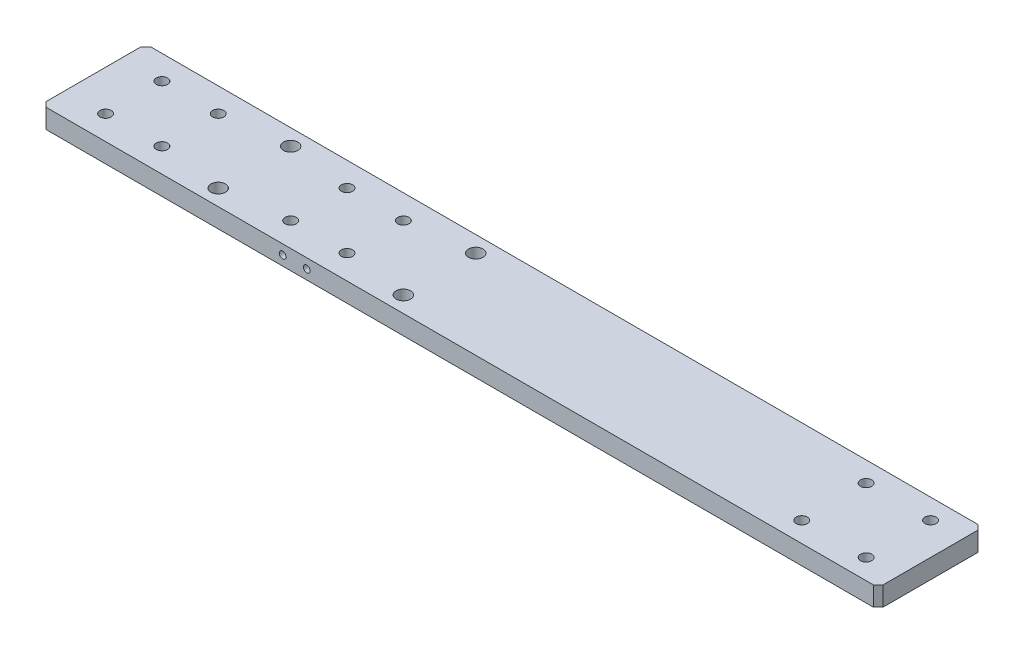
from build123d import *

# Parameters (mm, degrees)
SKETCH_2_W             = 520
SKETCH_2_H             = 65
EXTRUDE_1_DEPTH        = 12
HOLE_WIZARD_7_0_7_1_D  = 7
CHAMFER_1_SIZE         = 3
HOLE_WIZARD_9_0_9_2_D  = 9
HOLE_WIZARD_9_0_9_1_D  = 7
PATTERN_LINEAR_1_COUNT = 2
PATTERN_LINEAR_1_PITCH = 115
HOLE_WIZARD_9_0_9_3_D  = 9
HOLE_WIZARD_M5_1_D     = 4.2
HOLE_WIZARD_M5_1_DEPTH = 12.4
HOLE_WIZARD_M5_1_TIP   = 1.2618073
HOLE_WIZARD_M5_2_D     = 4.2
HOLE_WIZARD_M5_2_DEPTH = 12.4
HOLE_WIZARD_M5_2_TIP   = 1.2618073


with BuildPart() as part:
    # 草图2 → 凸台-拉伸1 (new body)
    with BuildSketch(Plane(origin=(0, 0, 0), x_dir=(1, 0, 0), z_dir=(0, 1, 0))):
        Rectangle(SKETCH_2_W, SKETCH_2_H)
    extrude(amount=EXTRUDE_1_DEPTH)

    # Ø7.0 (7) 直径孔1 (through all)
    with Locations(Plane.XZ):
        with Locations((240, -20), (200, -20), (200, 20), (240, 20)):
            Hole(HOLE_WIZARD_7_0_7_1_D / 2)

    # 倒角1
    chamfer_1_edges = [part.edges().sort_by_distance(p)[0] for p in [
        (260, 6, 32.5),
        (-260, 6, 32.5),
        (-260, 6, -32.5),
        (260, 6, -32.5),
    ]]
    chamfer(chamfer_1_edges, length=CHAMFER_1_SIZE)

    # Ø9.0 (9) 直径孔2 (through all)
    with Locations(Plane(origin=(0, 12, 0), x_dir=(1, 0, 0), z_dir=(0, 1, 0))):
        with Locations((-160, -22.5), (-160, 22.5)):
            Hole(HOLE_WIZARD_9_0_9_2_D / 2)

    # Ø9.0 (9) 直径孔1 (through all)
    with Locations(Plane(origin=(0, 12, 0), x_dir=(1, 0, 0), z_dir=(0, 1, 0))):
        with Locations((-235, -17.5), (-235, 17.5), (-200, -17.5), (-200, 17.5)):
            hole_wizard_9_0_9_1 = Hole(HOLE_WIZARD_9_0_9_1_D / 2)

    # 阵列(线性)1: Ø9.0 (9) 直径孔1 ×2
    with Locations(*[(i * PATTERN_LINEAR_1_PITCH, 0, 0) for i in range(1, PATTERN_LINEAR_1_COUNT)]):
        add(hole_wizard_9_0_9_1, mode=Mode.SUBTRACT)

    # Ø9.0 (9) 直径孔3 (through all)
    with Locations(Plane(origin=(0, 12, 0), x_dir=(1, 0, 0), z_dir=(0, 1, 0))):
        with Locations((-45, -22.5), (-45, 22.5)):
            Hole(HOLE_WIZARD_9_0_9_3_D / 2)

    # M5 螺纹孔1
    with Locations(Plane(origin=(0, 0, -32.5), x_dir=(-1, 0, 0), z_dir=(0, 0, -1))):
        with Locations((95, 6), (110, 6)):
            Hole(HOLE_WIZARD_M5_1_D / 2, depth=HOLE_WIZARD_M5_1_DEPTH)
            with Locations((0, 0, -(HOLE_WIZARD_M5_1_DEPTH + HOLE_WIZARD_M5_1_TIP / 2))):  # 118° drill point
                Cone(0, HOLE_WIZARD_M5_1_D / 2, HOLE_WIZARD_M5_1_TIP, mode=Mode.SUBTRACT)

    # M5 螺纹孔2
    with Locations(Plane.XY.offset(32.5)):
        with Locations((-95, 6), (-110, 6)):
            Hole(HOLE_WIZARD_M5_2_D / 2, depth=HOLE_WIZARD_M5_2_DEPTH)
            with Locations((0, 0, -(HOLE_WIZARD_M5_2_DEPTH + HOLE_WIZARD_M5_2_TIP / 2))):  # 118° drill point
                Cone(0, HOLE_WIZARD_M5_2_D / 2, HOLE_WIZARD_M5_2_TIP, mode=Mode.SUBTRACT)


solid = part.part
